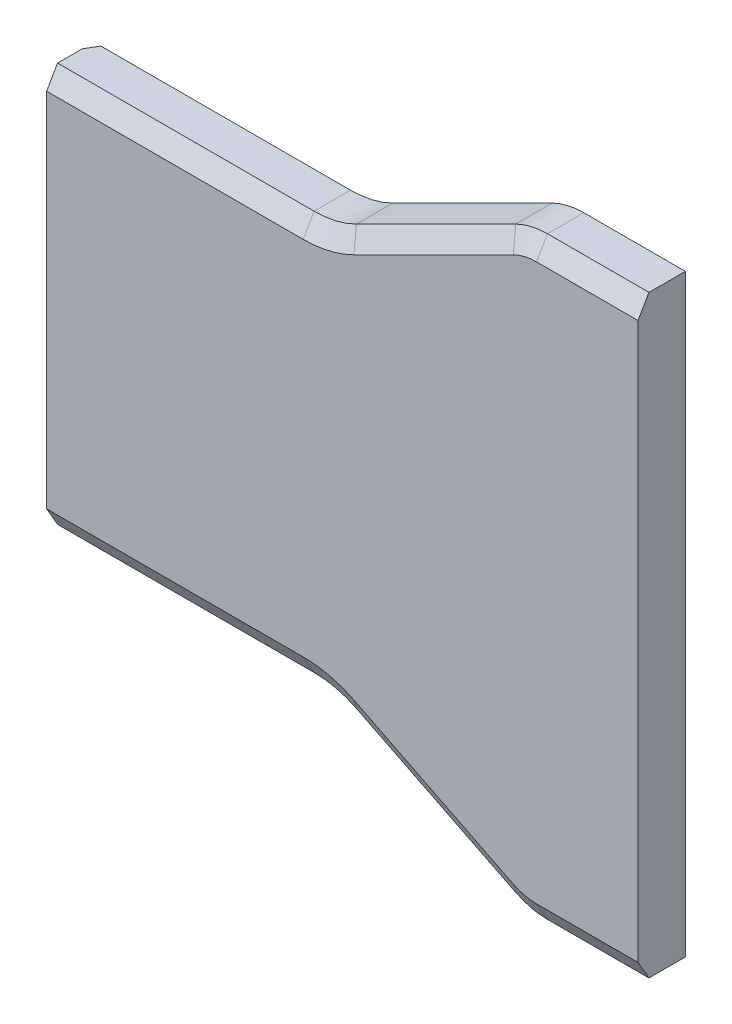
SolidWorks part; units mm, degrees
material "Q345 "
ref_plane "前视基准面" through (0, 0, 0) normal (0, 0, 1) x (1, 0, 0)
ref_plane "上视基准面" through (0, 0, 0) normal (0, 1, 0) x (1, 0, 0)
ref_plane "右视基准面" through (0, 0, 0) normal (1, 0, 0) x (0, 0, -1)
sketch "草图1" plane through (0, 0, 0) normal (0, 0, 1) x (1, 0, 0)
  line L4 (-305.5079, -251) -> (-322.918, -251)
  line L6 (-300, 0) -> (-322.918, 0)
  line L10 (-300, 0) -> (-280, 0)
  line L11 (-205.1487, 0) -> (-294.8513, 0) construction
  line L12 (-280, 0) -> (-280, -251)
  line L13 (-294.8513, -251) -> (-205.1487, -251) construction
  line L14 (-280, -251) -> (-305.5079, -251)
  line L15 (-421.5542, -209.9443) -> (-530, -209.9443)
  line L18 (-530, -41.0557) -> (-421.5542, -41.0557)
  line L22 (-530, -41.0557) -> (-530, -209.9443)
  line L24 (-205.1487, 0) -> (-294.8513, 0) construction
  line L30 (-403.6656, -214.1672) -> (-336.3344, -247.8328)
  line L31 (-403.6656, -36.8328) -> (-336.3344, -3.1672)
  line L36 (-530, -209.9443) -> (-421.5542, -209.9443) construction
  line L38 (-305.5079, -261) -> (-305.5079, -251) construction
  arc A14 (-336.3344, -247.8328) -> (-322.918, -251) centre (-322.918, -221) ccw construction
  arc A15 (-322.918, 0) -> (-336.3344, -3.1672) centre (-322.918, -30) ccw construction
  arc A16 (-403.6656, -214.1672) -> (-421.5542, -209.9443) centre (-421.5542, -249.9443) ccw construction
  arc A17 (-421.5542, -41.0557) -> (-403.6656, -36.8328) centre (-421.5542, -1.0557) ccw construction
  arc A18 (-336.3344, -247.8328) -> (-322.918, -251) centre (-322.918, -221) ccw
  arc A19 (-403.6656, -214.1672) -> (-421.5542, -209.9443) centre (-421.5542, -249.9443) ccw
  arc A20 (-322.918, 0) -> (-336.3344, -3.1672) centre (-322.918, -30) ccw
  arc A21 (-421.5542, -41.0557) -> (-403.6656, -36.8328) centre (-421.5542, -1.0557) ccw
  dimension "D1" = 20
extrude "凸台-拉伸1" add sketch "草图1" against normal blind 20
chamfer "倒角1" distance 8 angle 30 10 edges at (-301.459, -251, 0) (-329.8105, -250.1975, 0) (-301.459, 0, 0) (-370, -231, 0) (-370, -20, 0) (-475.7771, -209.9443, 0) (-412.3641, -211.0143, 0) (-475.7771, -41.0557, 0) (-412.3641, -39.9857, 0) (-329.8105, -0.8025, 0)
chamfer "倒角3" distance 5 angle 30 1 edges at (-530, -125.5, -20)
